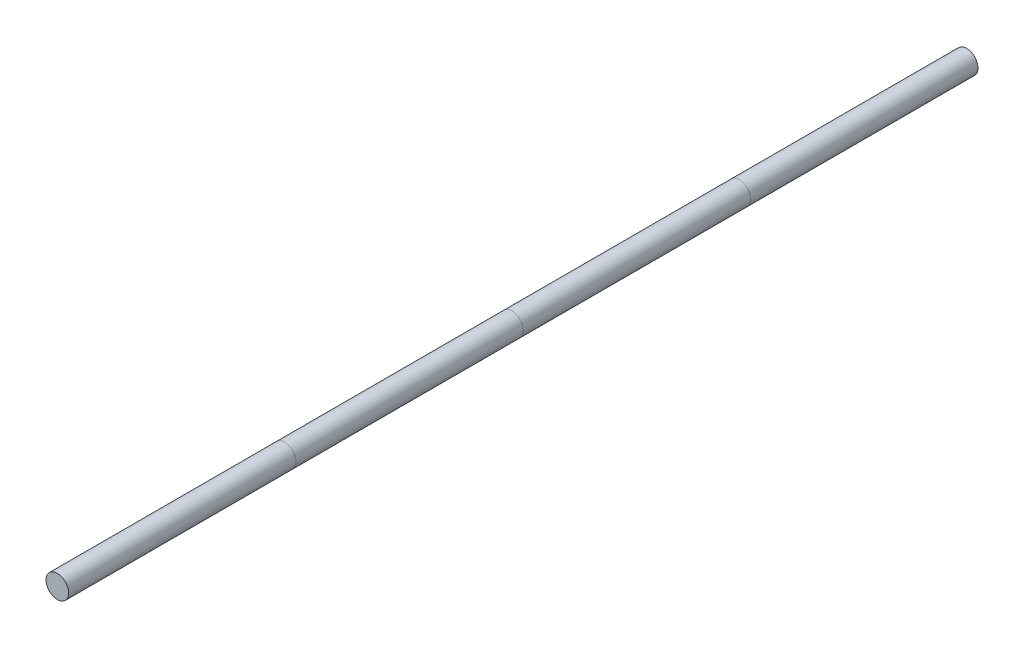
from build123d import *

# Parameters (mm, degrees)
SKETCH1_R           = 5
BOSS_EXTRUDE1_DEPTH = 400


with BuildPart() as part:
    # Sketch1 → Boss-Extrude1 (new body)
    with BuildSketch(Plane.XY):
        Circle(SKETCH1_R)
    extrude(amount=BOSS_EXTRUDE1_DEPTH)


solid = part.part
